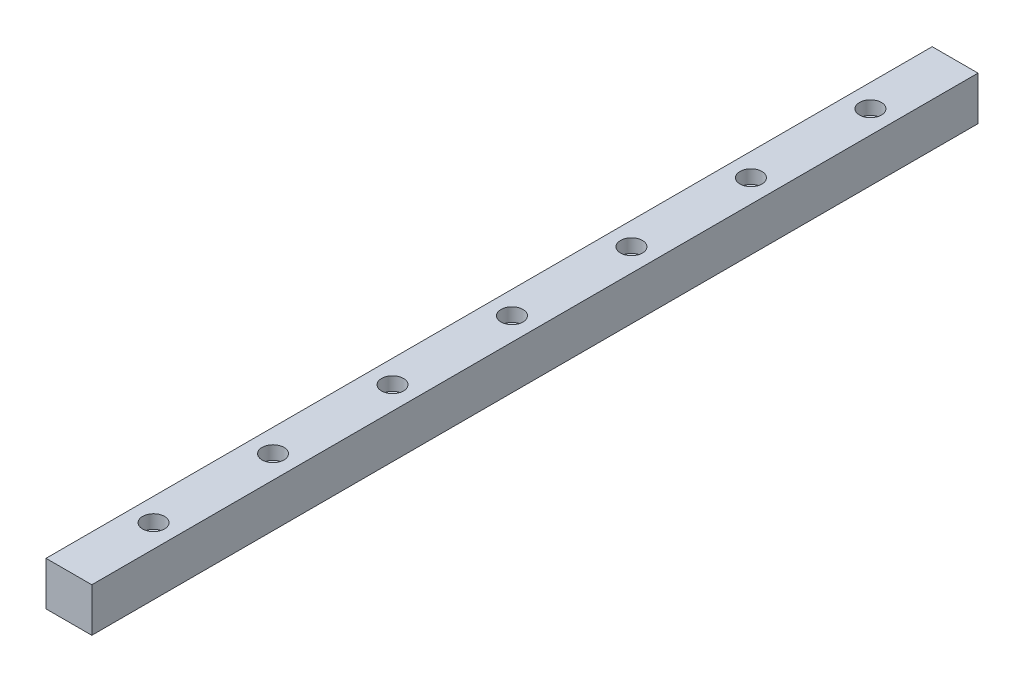
SolidWorks part; units mm, degrees
ref_plane "前视基准面" through (0, 0, 0) normal (0, 0, 1) x (1, 0, 0)
ref_plane "上视基准面" through (0, 0, 0) normal (0, 1, 0) x (1, 0, 0)
ref_plane "右视基准面" through (0, 0, 0) normal (1, 0, 0) x (0, 0, -1)
sketch "草图1" plane through (0, 0, 0) normal (0, 0, 1) x (1, 0, 0)
  line L1 (-11.5, 22) -> (11.5, 22)
  line L2 (-11.5, 22) -> (-11.5, 0)
  line L3 (-11.5, 0) -> (11.5, 0)
  line L4 (11.5, 22) -> (11.5, 0)
  dimension "D1" = 23
  dimension "D2" = 22
extrude "凸台-拉伸1" add sketch "草图1" along normal blind 445
hole_wizard "打孔尺寸(%根据)内六角圆柱头螺钉的类型1" positions "草图3" profile "草图2" counterbore size "M6" standard "GB" end condition through all
sketch "草图3" plane through (0, 22, 0) normal (0, 1, 0) x (1, 0, 0)
  line L0 (0, -445) -> (0, -433.4511) construction
  line L1 (11.5, -445) -> (-11.5, -445) construction
  point P0 (0, -402.5)
  dimension "D1" = 42.5
sketch "草图2" plane through (0, 22, 402.5) normal (1, 0, 0) x (0, 0, 1)
  line L0 (0, 0) -> (0, 22)
  line L1 (0, 22) -> (3.3, 22)
  line L3 (3.3, 22) -> (3.3, 6.8)
  line L4 (3.3, 6.8) -> (5.5, 6.8)
  line L5 (5.5, 6.8) -> (5.5, 0)
  line L7 (5.5, 0) -> (0, 0)
  line L11 (0, -6.35) -> (0, 107.95) construction
  dimension "通孔孔直径" = 6.6
  dimension "通孔孔深度" = 22
  dimension "柱形沉头孔直径" = 11
  dimension "柱形沉头孔深度" = 6.8
pattern_linear "阵列(线性)1" count 8 spacing 60 along (0, 0, -1) of "打孔尺寸(%根据)内六角圆柱头螺钉的类型1"
